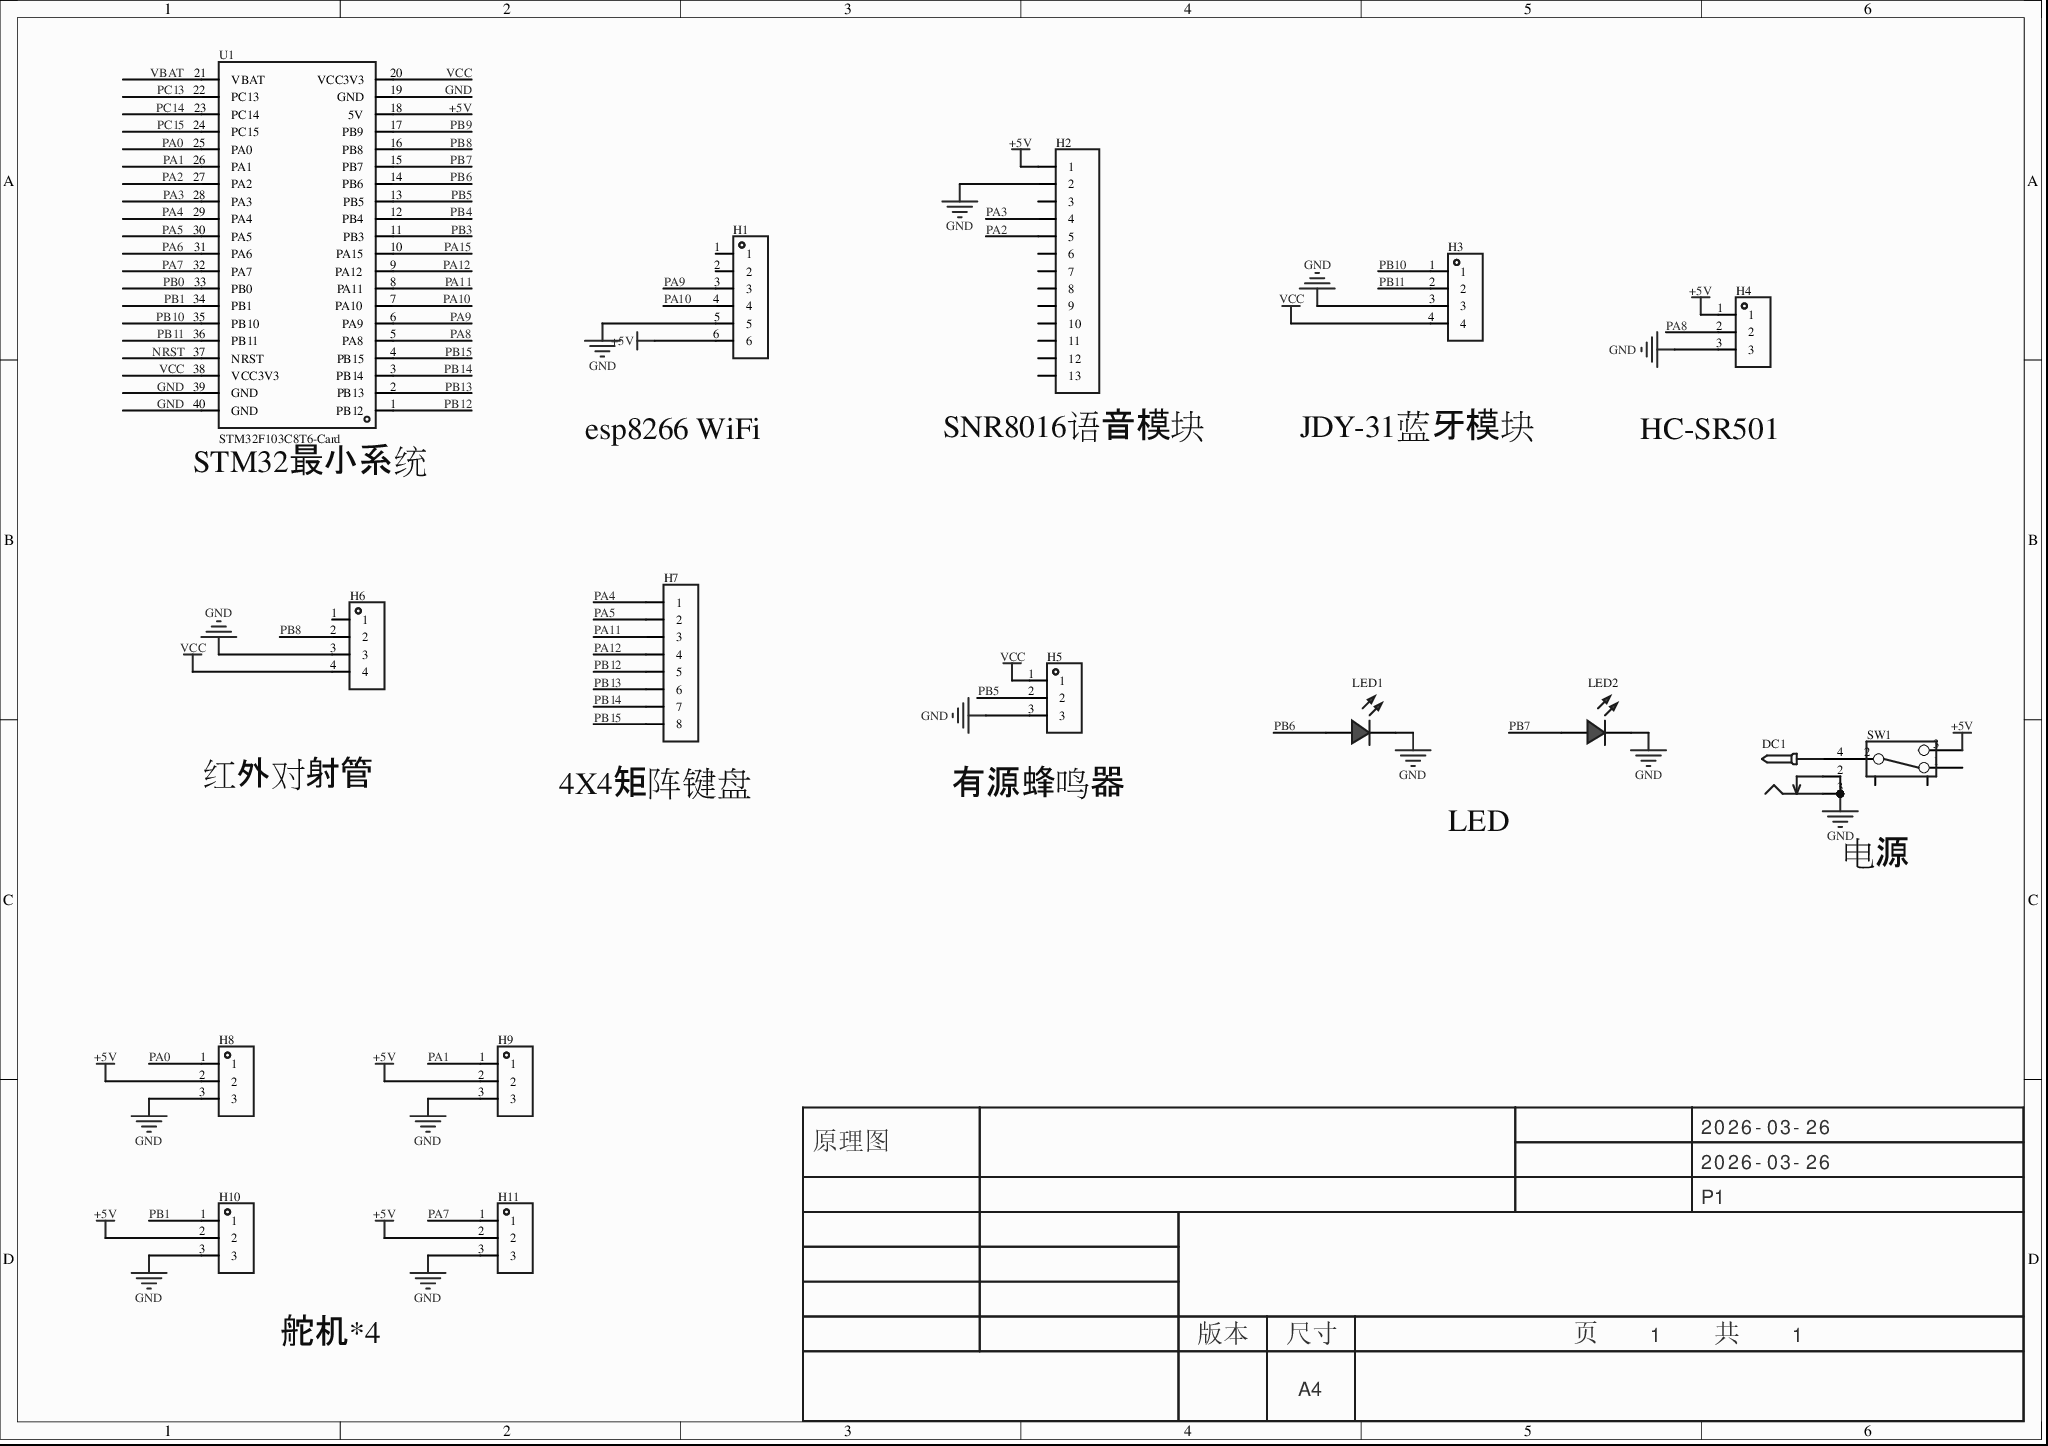
[diagram p0: MISC52050-3.schdoc]
# Altium project MISC52050-2.PrjPcb
1 sheet, 16 parts. Net scope: global (net labels, ports and power ports of the same name join across sheets).
Board file: MISC52050.pcbdoc

## Sheet MISC52050-3.schdoc
size 297 x 209 mm; Version: V1.0; @Project Name: MISC52050; @Page Count: 1; @Update Date: 2026-03-26; @Create Date: 2026-03-26; @Schematic Name: MISC52050; @Page No: 1; @Create Time: 18:58:15; @Update Time: 22:44:58; @Board Name: MISC52050

### Parts
DC1  (no value)  [DC-2.0]
H1  (no value)  [HDR-TH_6P-P2.54-V-F]
H2  (no value)  [HDR-TH_13P-P2.54-V-F]
H3  (no value)  [HDR-TH_4P-P2.54-V-F]
H4  (no value)  [HDR-TH_3P-P2.54-V-F]
H5  (no value)  [HDR-TH_3P-P2.54-V-F]
H6  (no value)  [HDR-TH_4P-P2.54-V-F]
H7  (no value)  [HDR-TH_8P-P2.54-V-F-1]
H8  (no value)  [HDR-TH_3P-P2.54-V-F]
H9  (no value)  [HDR-TH_3P-P2.54-V-F]
H10  (no value)  [HDR-TH_3P-P2.54-V-F]
H11  (no value)  [HDR-TH_3P-P2.54-V-F]
LED1  (no value)  [LED-TH_5mm]
LED2  (no value)  [LED-TH_5mm]
SW1  (no value)  [拨动开关]
U1  STM32F103C8T6-Card  [CONN-TH_L53.3-W22.9_STM32F103C8T6-CARD]

### Nets
+5V: H1.6 H2.1 H4.1 H8.2 H9.2 H10.2 H11.2 SW1.3 U1.18(5V)
GND: DC1.2 DC1.3 H1.5 H2.2 H3.3 H4.3 H5.3 H6.3 H8.3 H9.3 H10.3 H11.3 LED1.2(A) LED2.2(A) U1.19(GND) U1.39(GND) U1.40(GND)
VCC: H3.4 H5.1 H6.4 U1.20(VCC3V3) U1.38(VCC3V3)
NRST: U1.37(NRST)
PA0: H8.1 U1.25(PA0)
PA1: H9.1 U1.26(PA1)
PA2: H2.5 U1.27(PA2)
PA3: H2.4 U1.28(PA3)
PA4: H7.1 U1.29(PA4)
PA5: H7.2 U1.30(PA5)
PA6: U1.31(PA6)
PA7: H11.1 U1.32(PA7)
PA8: H4.2 U1.5(PA8)
PA9: H1.3 U1.6(PA9)
PA10: H1.4 U1.7(PA10)
PA11: H7.3 U1.8(PA11)
PA12: H7.4 U1.9(PA12)
PA15: U1.10(PA15)
PB0: U1.33(PB0)
PB1: H10.1 U1.34(PB1)
PB3: U1.11(PB3)
PB4: U1.12(PB4)
PB5: H5.2 U1.13(PB5)
PB6: LED1.1(C) U1.14(PB6)
PB7: LED2.1(C) U1.15(PB7)
PB8: H6.2 U1.16(PB8)
PB9: U1.17(PB9)
PB10: H3.1 U1.35(PB10)
PB11: H3.2 U1.36(PB11)
PB12: H7.5 U1.1(PB12)
PB13: H7.6 U1.2(PB13)
PB14: H7.7 U1.3(PB14)
PB15: H7.8 U1.4(PB15)
PC13: U1.22(PC13)
PC14: U1.23(PC14)
PC15: U1.24(PC15)
VBAT: U1.21(VBAT)
NetDC1_4: DC1.4 SW1.2

Not connected (* = marked no-connect by the designer): H1 1 2; H2 3 6 7 8 9 10 11 12 13; H6 1; SW1 1 4 5

### Notes on the sheet
- (near U1) STM32最小系统
- esp8266 WiFi
- (near H2) SNR8016语音模块
- JDY-31蓝牙模块
- (near H4) HC-SR501
- 红外对射管
- (near H7) 4X4矩阵键盘
- (near H5) 有源蜂鸣器
- LED
- 电源
- 舵机*4
- 2026-03-26
- 原理图
- P1
- 版本
- 尺寸
- A4
- 页    1    共    1

### Library data of the parts
DC1 = DC-005_2.0: Symbol: DC电源接口; 3D Model: f5f20b8a2308479b936ba3c2698865bb0819f05c4eef4c71ace90d822a990e87; 3D Model Transform: 372.05,551.18,582.68,90,0,0,137.8,0,-149.61; ConvertToPcb: yes; ModelName: DC-IN-TH_DC-5520-1; Device: DC-005_2.0; Supplier Footprint: 插件; AddInBom: yes; FootprintName: DC-2.0
H1 = HDR-F_2.54_1x6P: Symbol: Header-Female-2.54_1x6; 3D Model: 0f5bcf94dcda47d085f24cdca1696fe9; 3D Model Transform: 619.684,94.488,0,0,0,0,0,0,-125.984; ConvertToPcb: yes; Device: HDR-F_2.54_1x6P; Supplier Part: C40877; Supplier Footprint: 插件; AddInBom: yes; FootprintName: HDR-TH_6P-P2.54-V-F; ModelName: HDR-TH_6P-P2.54-V-F
H2 = HDR-F_2.54_1x13P: ConvertToPcb: yes; ModelId: d941d8cd8ae04597bbb25c940a0252b50819f05c4eef4c71ace90d822a990e87; ModelName: HDR-TH_13P-P2.54-F-LI-1X13P; ModelTransform: 98.425,1315.74548,0,90,0,0,0,0,-125.984; Symbol: HDR-F_2.54_1x13P; Device: HDR-F_2.54_1x13P; AddInBom: yes; SupplierPart: C52709; Supplier Footprint: 插件; FootprintName: HDR-TH_13P-P2.54-V-F
H3 H6 = HDR-F_2.54_1x4P: Symbol: 2.54-1*4P母; 3D Model: d187812051054f85879fcaa51a310d8e0819f05c4eef4c71ace90d822a990e87; 3D Model Transform: 419.6842,98.464,0,0,0,0,0,0,-118.11; ConvertToPcb: yes; Device: HDR-F_2.54_1x4P; Supplier Part: C2718488; Supplier Footprint: 插件; AddInBom: yes; FootprintName: HDR-TH_4P-P2.54-V-F; ModelName: HDR-TH_4P-P2.54-V-F
H4 H5 H8-H11 = HDR-F_2.54_1x3P: Symbol: PM254V-11-03-H85; 3D Model: f3b3cc5aae9641bf9e56fc160cef875b; 3D Model Transform: 299.9994,100,0,0,0,0,0,0,-118.11; ConvertToPcb: yes; ModelName: HDR2.54-F-LI-1X3P; Device: HDR-F_2.54_1x3P; Supplier Part: C541850; Supplier Footprint: 插件; AddInBom: yes; FootprintName: HDR-TH_3P-P2.54-V-F
H7 = HDR-F_2.54_1x8P: Symbol: Header-Female-2.54_1x8; 3D Model: 0f7e4d9227ef4fa08d5469c22cc70cdb; 3D Model Transform: 799.99844,100,0,0,0,0,0,0,-118.11; AddInBom: yes; ModelName: HDR-F-2.54_1x8; Device: HDR-F_2.54_1x8P; Supplier Part: C27438; Supplier Footprint: 插件; ConvertToPcb: yes; FootprintName: HDR-TH_8P-P2.54-V-F-1
LED1 LED2 = LED_TH-R_5mm: ConvertToPcb: yes; ModelId: fe9cea1bdf7642cd8d9a5077ed0e2b580819f05c4eef4c71ace90d822a990e87; ModelName: LED-TH_BD5.9-P2.54-RD_RED; ModelTransform: 222.16,238.98,581.81,180,0,0,-6,0,-220; Symbol: LED_TH-R; Device: LED_TH-R_5mm; AddInBom: yes; FootprintName: LED-TH_5mm; Supplier Footprint: 插件
SW1 = 拨动开关_正: ConvertToPcb: yes; ModelId: 4321fe59a4074cbfb4989553f297c68f0819f05c4eef4c71ace90d822a990e87; ModelName: SW-TH_SS-12D02-VG4; ModelTransform: 370.09,208.7,472.35,0,0,0,0,0,-110; Symbol: 拨动开关; Device: 拨动开关_正; AddInBom: yes; Supplier Footprint: 插件; FootprintName: 拨动开关
U1 = STM32F103C8T6-Card: AddInBom: yes; Symbol: STM32F103C8T6-CARD; Device: STM32F103C8T6-Card; LCSC Part Name: STM32F103C8T6-Card; SupplierPart: C9900077949; ManufacturerPart: STM32F103C8T6-Card; Supplier Footprint: 插件; Supplier: LCSC; ConvertToPcb: yes; FootprintName: CONN-TH_L53.3-W22.9_STM32F103C8T6-CARD